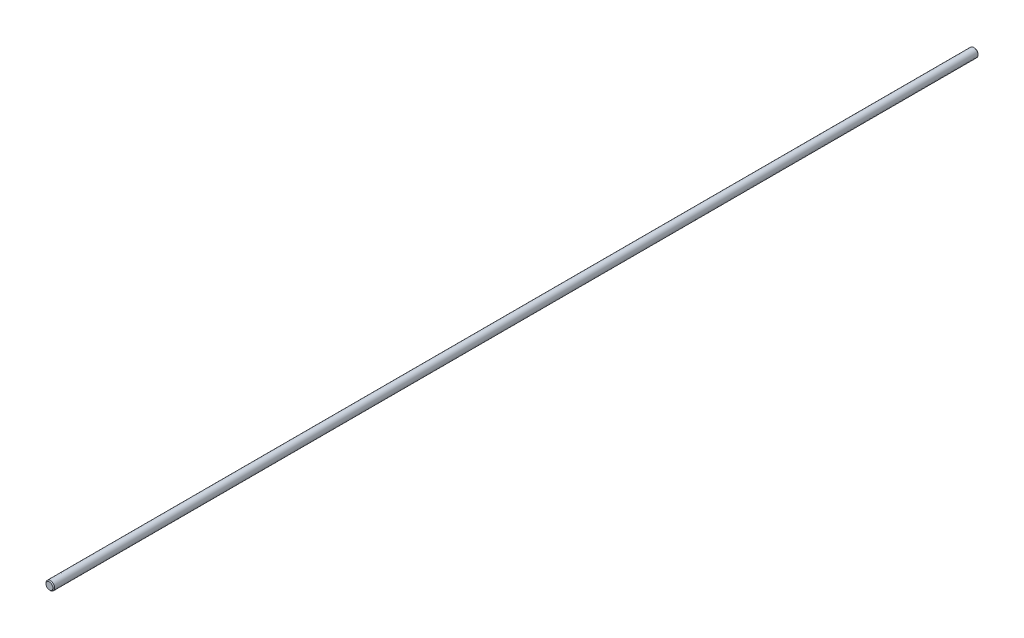
from build123d import *

# Parameters (mm, degrees)
SKETCH_1_R      = 10
EXTRUDE_1_DEPTH = 2135
CHAMFER_1_SIZE  = 2


with BuildPart() as part:
    # 草图1 → 凸台-拉伸1 (new body)
    with BuildSketch(Plane.XY):
        Circle(SKETCH_1_R)
    extrude(amount=EXTRUDE_1_DEPTH)

    # 倒角1
    chamfer_1_edges = [part.edges().sort_by_distance(p)[0] for p in [
        (-10, 0, 0),
        (-10, 0, 2135),
    ]]
    chamfer(chamfer_1_edges, length=CHAMFER_1_SIZE)


solid = part.part
